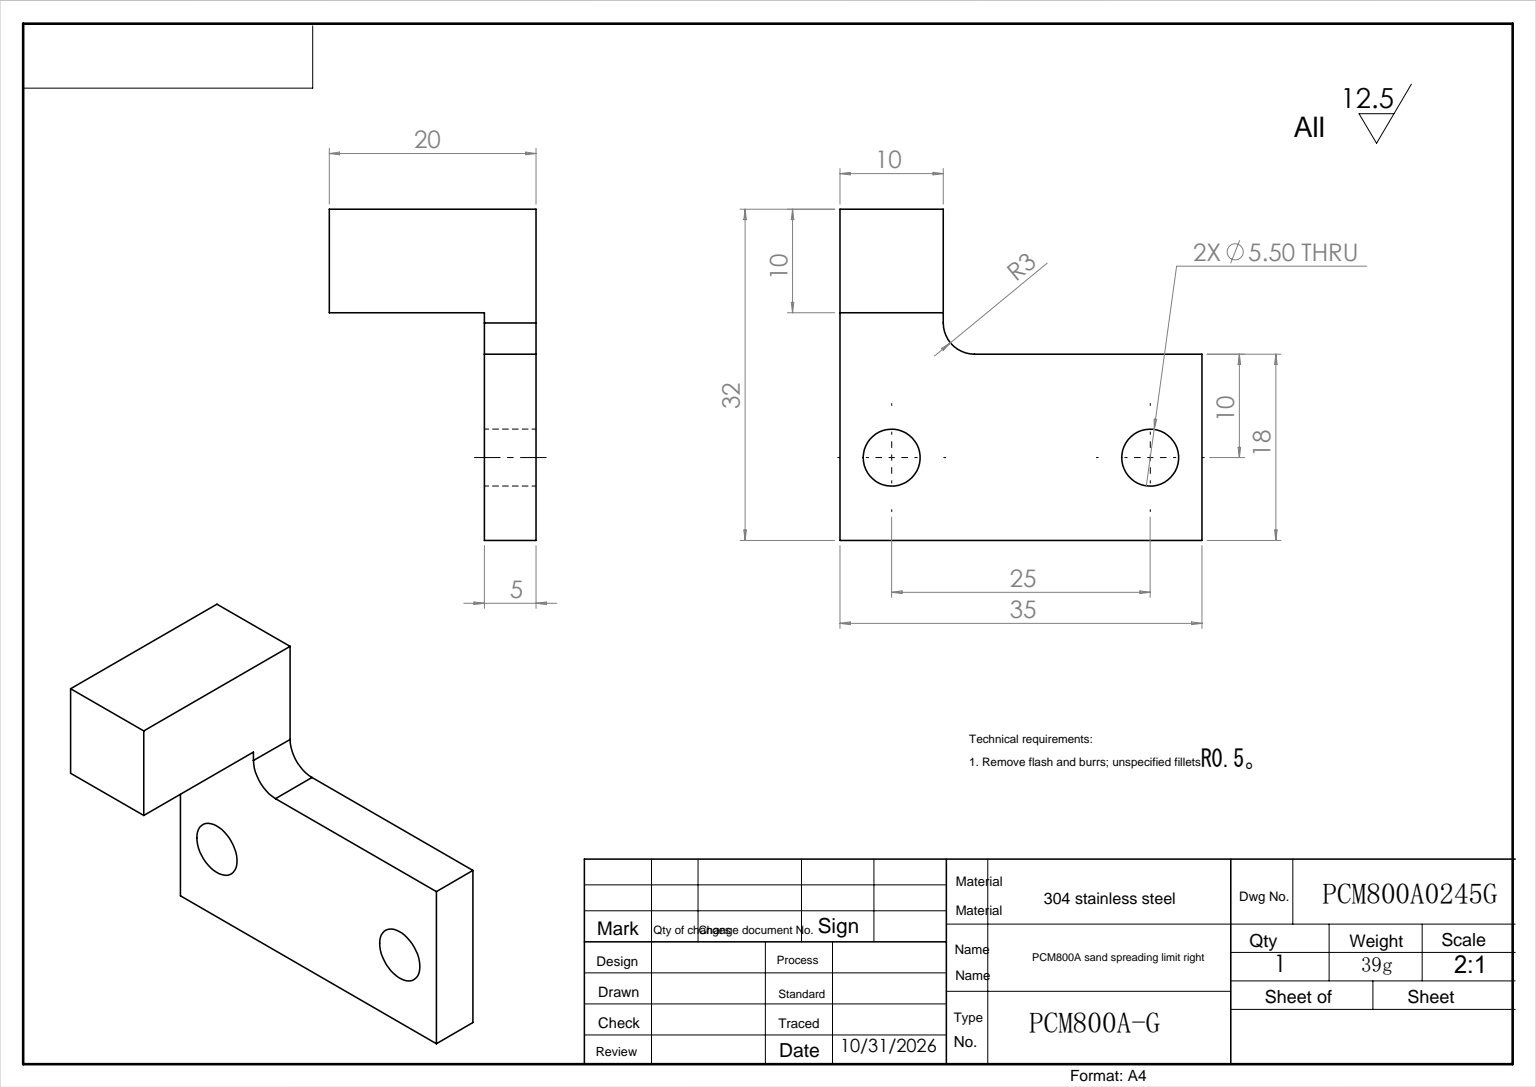
from build123d import *

# Parameters (mm, degrees)
EXTRUDE_1_DEPTH     = 5
SKETCH_5_W          = 10
SKETCH_5_H          = 10
EXTRUDE_3_DEPTH     = 20
SKETCH_4_R          = 2.75
CUT_EXTRUDE_1_DEPTH = 20


with BuildPart() as part:
    # 草图1 → 凸台-拉伸1 (new body)
    with BuildSketch(Plane.XY):
        with BuildLine():
            Line((0, 0), (35, 0))
            Line((35, 0), (35, 18))
            Line((35, 18), (13, 18))
            ThreePointArc((13, 18), (10.878679656, 18.878679656), (10, 21))
            Line((10, 21), (10, 22))
            Line((10, 22), (0, 22))
            Line((0, 22), (0, 0))
        make_face()
    extrude(amount=EXTRUDE_1_DEPTH)

    # 草图5 → 凸台-拉伸3 (add)
    with BuildSketch(Plane(origin=(0, 0, 0), x_dir=(-1, 0, 0), z_dir=(0, 0, -1))):
        with Locations((-5, 27)):
            Rectangle(SKETCH_5_W, SKETCH_5_H)
    extrude(amount=-EXTRUDE_3_DEPTH)

    # 草图4 → 切除-拉伸1 (cut)
    with BuildSketch(Plane(origin=(0, 0, 0), x_dir=(-1, 0, 0), z_dir=(0, 0, -1))):
        with Locations((-30, 8)):
            Circle(SKETCH_4_R)
        with Locations((-5, 8)):
            Circle(SKETCH_4_R)
    extrude(amount=-CUT_EXTRUDE_1_DEPTH, mode=Mode.SUBTRACT)


solid = part.part
